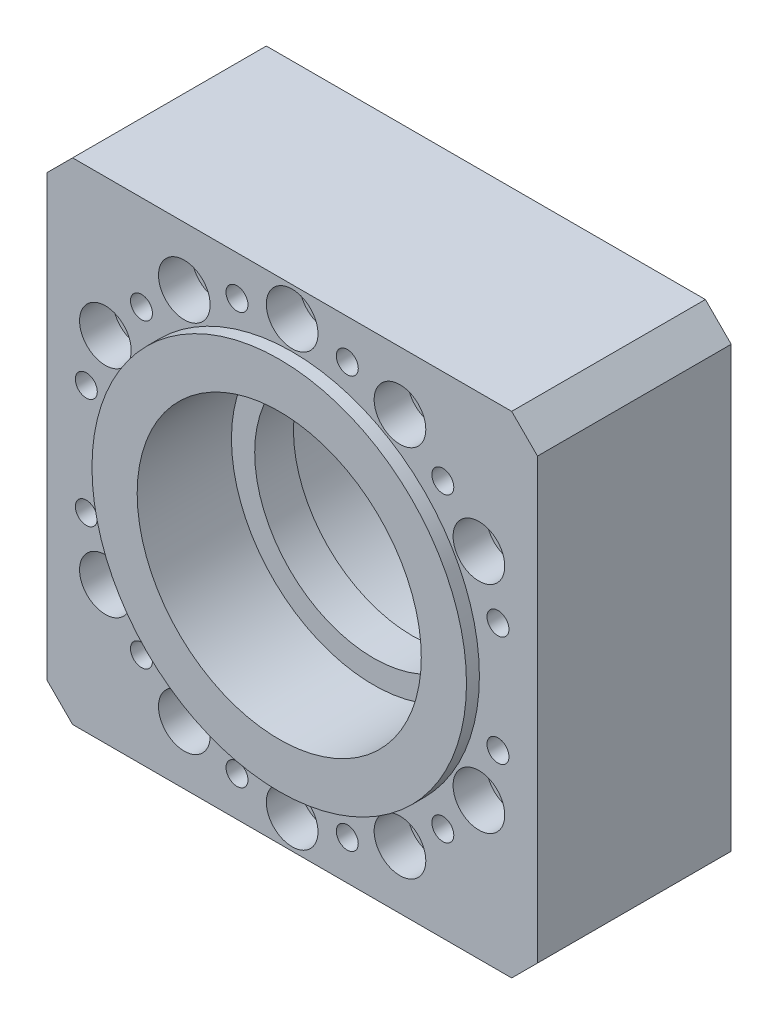
from build123d import *

# Parameters (mm, degrees)
SKETCH1_W                                            = 190
SKETCH1_H                                            = 190
BOSS_EXTRUDE1_DEPTH                                  = 75
SKETCH2_R                                            = 33
CUT_EXTRUDE1_DEPTH                                   = 154.866825534
HOLE_SIZE_PER_SOCKET_HEAD_CAP_SCREW_TYPE_D           = 13.5
HOLE_SIZE_PER_SOCKET_HEAD_CAP_SCREW_TYPE_CBORE_D     = 20
HOLE_SIZE_PER_SOCKET_HEAD_CAP_SCREW_TYPE_CBORE_DEPTH = 13
CIRPATTERN1_COUNT                                    = 12
CHAMFER1_SIZE                                        = 10
CIRPATTERN2_COUNT                                    = 12
SKETCH14_R                                           = 40
CUT_EXTRUDE5_DEPTH                                   = 50
CUT_EXTRUDE6_START                                   = -50
SKETCH15_R                                           = 40
CUT_EXTRUDE6_DEPTH                                   = 50
SKETCH17_R                                           = 75
SKETCH17_R_2                                         = 55
BOSS_EXTRUDE3_DEPTH                                  = 10
SKETCH19_R                                           = 45
CUT_EXTRUDE8_DEPTH                                   = 25
SKETCH20_R                                           = 55
CUT_EXTRUDE9_DEPTH                                   = 159.981130956
BOSS_EXTRUDE4_START                                  = -35
SKETCH21_R                                           = 55
SKETCH21_R_2                                         = 42.5
BOSS_EXTRUDE4_DEPTH                                  = 35
CHAMFER3_SIZE                                        = 1
CIRPATTERN3_COUNT                                    = 4
CUT_EXTRUDE11_START                                  = -2.5
SKETCH24_OUTSIDE_W                                   = 248.364
SKETCH24_OUTSIDE_H                                   = 248.364
SKETCH24_OUTSIDE_R                                   = 73.15
CUT_EXTRUDE11_DEPTH                                  = 4.7
SKETCH25_R                                           = 55
CUT_EXTRUDE12_DEPTH                                  = 159.981130956
BOSS_EXTRUDE5_START                                  = -31.5
SKETCH26_R                                           = 55
SKETCH26_R_2                                         = 40
BOSS_EXTRUDE5_DEPTH                                  = 15
BOSS_EXTRUDE6_START                                  = 5
SKETCH27_R                                           = 72.5
SKETCH27_R_2                                         = 55
BOSS_EXTRUDE6_DEPTH                                  = 5
SKETCH28_R                                           = 46
CUT_EXTRUDE13_DEPTH                                  = 145.610684253


with BuildPart() as part:
    # Sketch1 → Boss-Extrude1 (new body)
    with BuildSketch(Plane.XY):
        Rectangle(SKETCH1_W, SKETCH1_H)
    extrude(amount=BOSS_EXTRUDE1_DEPTH)

    # Sketch2 → Cut-Extrude1 (cut, through all)
    with BuildSketch(Plane.XY.offset(75)):
        Circle(SKETCH2_R)
    extrude(amount=-CUT_EXTRUDE1_DEPTH, mode=Mode.SUBTRACT)

    # Hole size per socket head cap screw type1 (through all)
    with Locations(Plane.XY.offset(75)):
        with Locations((0, 83.5)):
            hole_size_per_socket_head_cap_screw_type = CounterBoreHole(HOLE_SIZE_PER_SOCKET_HEAD_CAP_SCREW_TYPE_D / 2, HOLE_SIZE_PER_SOCKET_HEAD_CAP_SCREW_TYPE_CBORE_D / 2, HOLE_SIZE_PER_SOCKET_HEAD_CAP_SCREW_TYPE_CBORE_DEPTH)

    # CirPattern1: Hole size per socket head cap screw type1 ×12 about axis, 2 skipped
    cirpattern1_axis = Axis((0, 0, 0), (0, 0, -1))
    add([hole_size_per_socket_head_cap_screw_type.rotate(cirpattern1_axis, i * 360 / CIRPATTERN1_COUNT) for i in range(1, CIRPATTERN1_COUNT) if i not in (3, 9)], mode=Mode.SUBTRACT)

    # Chamfer1
    chamfer1_edges = [part.edges().sort_by_distance(p)[0] for p in [
        (-95, 95, 37.5),
        (95, 95, 37.5),
        (95, -95, 37.5),
        (-95, -95, 37.5),
    ]]
    chamfer(chamfer1_edges, length=CHAMFER1_SIZE)

    # Sketch10 → M10 Tapped Hole1 (revolve, cut)
    with BuildSketch(Plane(origin=(21.352571221, 79.688880669, 75), x_dir=(0, -1, 0), z_dir=(1, 0, 0))):
        Polygon((0, 0), (0, 24.553657631), (4.25, 22), (4.25, 0), align=None)
    m10_tapped_hole1 = revolve(axis=Axis((21.352571221, 79.688880669, 81.35), (0, 0, -1)), mode=Mode.SUBTRACT)

    # CirPattern2: M10 Tapped Hole1 ×12 about axis
    cirpattern2_axis = Axis((0, 0, 0), (0, 0, 1))
    for i in range(1, CIRPATTERN2_COUNT):
        add(m10_tapped_hole1.rotate(cirpattern2_axis, i * 360 / CIRPATTERN2_COUNT), mode=Mode.SUBTRACT)

    # Sketch14 → Cut-Extrude5 (cut)
    with BuildSketch(Plane(origin=(0, 0, 0), x_dir=(-1, 0, 0), z_dir=(0, 0, -1))):
        Circle(SKETCH14_R)
    extrude(amount=-CUT_EXTRUDE5_DEPTH, mode=Mode.SUBTRACT)

    # Sketch15 → Cut-Extrude6 (cut)
    with BuildSketch(Plane.XY.offset(75).offset(CUT_EXTRUDE6_START)):
        with Locations(Location((0, 0, 0), (0, 0, 180))):
            Circle(SKETCH15_R)
    extrude(amount=CUT_EXTRUDE6_DEPTH, mode=Mode.SUBTRACT)

    # Sketch17 → Boss-Extrude3 (add)
    with BuildSketch(Plane(origin=(0, 0, 0), x_dir=(-1, 0, 0), z_dir=(0, 0, -1))):
        Circle(SKETCH17_R)
        Circle(SKETCH17_R_2, mode=Mode.SUBTRACT)
    extrude(amount=BOSS_EXTRUDE3_DEPTH)

    # Sketch19 → Cut-Extrude8 (cut)
    with BuildSketch(Plane.XY.offset(75)):
        Circle(SKETCH19_R)
    extrude(amount=-CUT_EXTRUDE8_DEPTH, mode=Mode.SUBTRACT)

    # Sketch20 → Cut-Extrude9 (cut, through all)
    with BuildSketch(Plane.XY.offset(75)):
        Circle(SKETCH20_R)
    extrude(amount=-CUT_EXTRUDE9_DEPTH, mode=Mode.SUBTRACT)

    # Sketch21 → Boss-Extrude4 (add)
    with BuildSketch(Plane(origin=(0, 0, -10), x_dir=(-1, 0, 0), z_dir=(0, 0, -1)).offset(BOSS_EXTRUDE4_START)):
        with Locations(Location((0, 0, 0), (0, 0, 180))):
            Circle(SKETCH21_R)
        Circle(SKETCH21_R_2, mode=Mode.SUBTRACT)
    extrude(amount=BOSS_EXTRUDE4_DEPTH)

    # Chamfer3
    chamfer3_edges = [part.edges().sort_by_distance(p)[0] for p in [
        (75, 0, -10),
    ]]
    chamfer(chamfer3_edges, length=CHAMFER3_SIZE)

    # Sketch23 → M6 Tapped Hole1 (revolve, cut)
    with BuildSketch(Plane(origin=(0, 63.25, -10), x_dir=(0, 1, 0), z_dir=(1, 0, 0))):
        Polygon((0, 0), (0, 16.502151548), (2.5, 15), (2.5, 0), align=None)
    m6_tapped_hole1 = revolve(axis=Axis((0, 63.25, -16.35), (0, 0, 1)), mode=Mode.SUBTRACT)

    # CirPattern3: M6 Tapped Hole1 ×4 about axis
    cirpattern3_axis = Axis((0, 0, 0), (0, 0, 1))
    for i in range(1, CIRPATTERN3_COUNT):
        add(m6_tapped_hole1.rotate(cirpattern3_axis, i * 360 / CIRPATTERN3_COUNT), mode=Mode.SUBTRACT)

    # Sketch24 outside → Cut-Extrude11 (cut)
    with BuildSketch(Plane(origin=(0, 0, -10), x_dir=(-1, 0, 0), z_dir=(0, 0, -1)).offset(CUT_EXTRUDE11_START)):
        Rectangle(SKETCH24_OUTSIDE_W, SKETCH24_OUTSIDE_H)
        Circle(SKETCH24_OUTSIDE_R, mode=Mode.SUBTRACT)
    extrude(amount=-CUT_EXTRUDE11_DEPTH, mode=Mode.SUBTRACT)

    # Sketch25 → Cut-Extrude12 (cut, through all)
    with BuildSketch(Plane.XY.offset(75)):
        Circle(SKETCH25_R)
    extrude(amount=-CUT_EXTRUDE12_DEPTH, mode=Mode.SUBTRACT)

    # Sketch26 → Boss-Extrude5 (add)
    with BuildSketch(Plane.XY.offset(75).offset(BOSS_EXTRUDE5_START)):
        Circle(SKETCH26_R)
        Circle(SKETCH26_R_2, mode=Mode.SUBTRACT)
    extrude(amount=-BOSS_EXTRUDE5_DEPTH)

    # Sketch27 → Boss-Extrude6 (add)
    with BuildSketch(Plane.XY.offset(75).offset(BOSS_EXTRUDE6_START)):
        Circle(SKETCH27_R)
        Circle(SKETCH27_R_2, mode=Mode.SUBTRACT)
    extrude(amount=-BOSS_EXTRUDE6_DEPTH)

    # Sketch28 → Cut-Extrude13 (cut, through all)
    with BuildSketch(Plane.XY.offset(43.5)):
        Circle(SKETCH28_R)
    extrude(amount=-CUT_EXTRUDE13_DEPTH, mode=Mode.SUBTRACT)


solid = part.part
